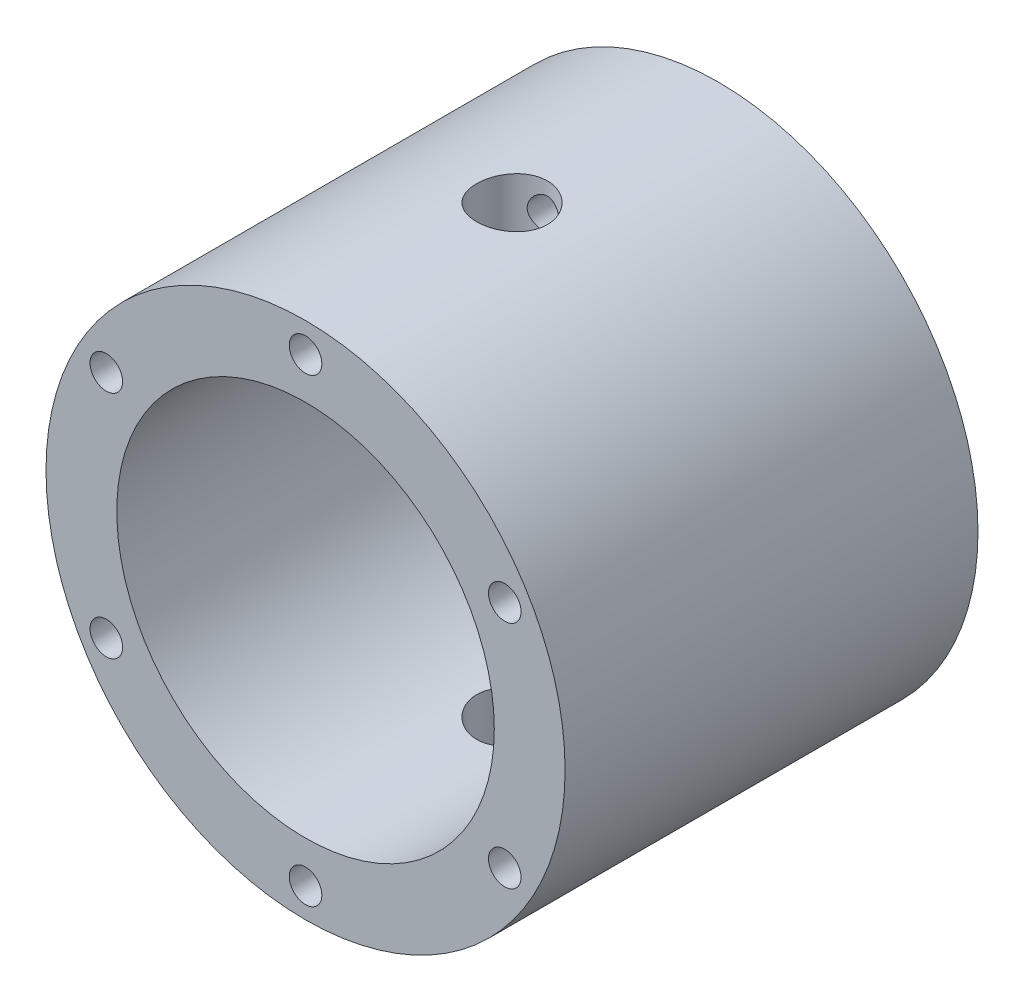
from build123d import *

# Parameters (mm, degrees)
SKETCH1_R           = 110
SKETCH1_R_2         = 80
SKETCH1_R_3         = 6.9
BOSS_EXTRUDE1_DEPTH = 175
SKETCH2_R           = 15
CUT_EXTRUDE1_DEPTH  = 1000


with BuildPart() as part:
    # Sketch1 → Boss-Extrude1 (new body)
    with BuildSketch(Plane.XY):
        Circle(SKETCH1_R)
        Circle(SKETCH1_R_2, mode=Mode.SUBTRACT)
        with Locations((0, 97.5)):
            Circle(SKETCH1_R_3, mode=Mode.SUBTRACT)
        with Locations((84.437476869, 48.75)):
            Circle(SKETCH1_R_3, mode=Mode.SUBTRACT)
        with Locations((84.437476869, -48.75)):
            Circle(SKETCH1_R_3, mode=Mode.SUBTRACT)
        with Locations((0, -97.5)):
            Circle(SKETCH1_R_3, mode=Mode.SUBTRACT)
        with Locations((-84.437476869, -48.75)):
            Circle(SKETCH1_R_3, mode=Mode.SUBTRACT)
        with Locations((-84.437476869, 48.75)):
            Circle(SKETCH1_R_3, mode=Mode.SUBTRACT)
    extrude(amount=BOSS_EXTRUDE1_DEPTH)

    # Sketch2 → Cut-Extrude1 (cut, symmetric)
    with BuildSketch(Plane(origin=(0, 0, 0), x_dir=(1, 0, 0), z_dir=(0, 1, 0))):
        with Locations(Location((0, -87.5, 0), (0, 0, 270))):
            Circle(SKETCH2_R)
    extrude(amount=CUT_EXTRUDE1_DEPTH, both=True, mode=Mode.SUBTRACT)


solid = part.part
